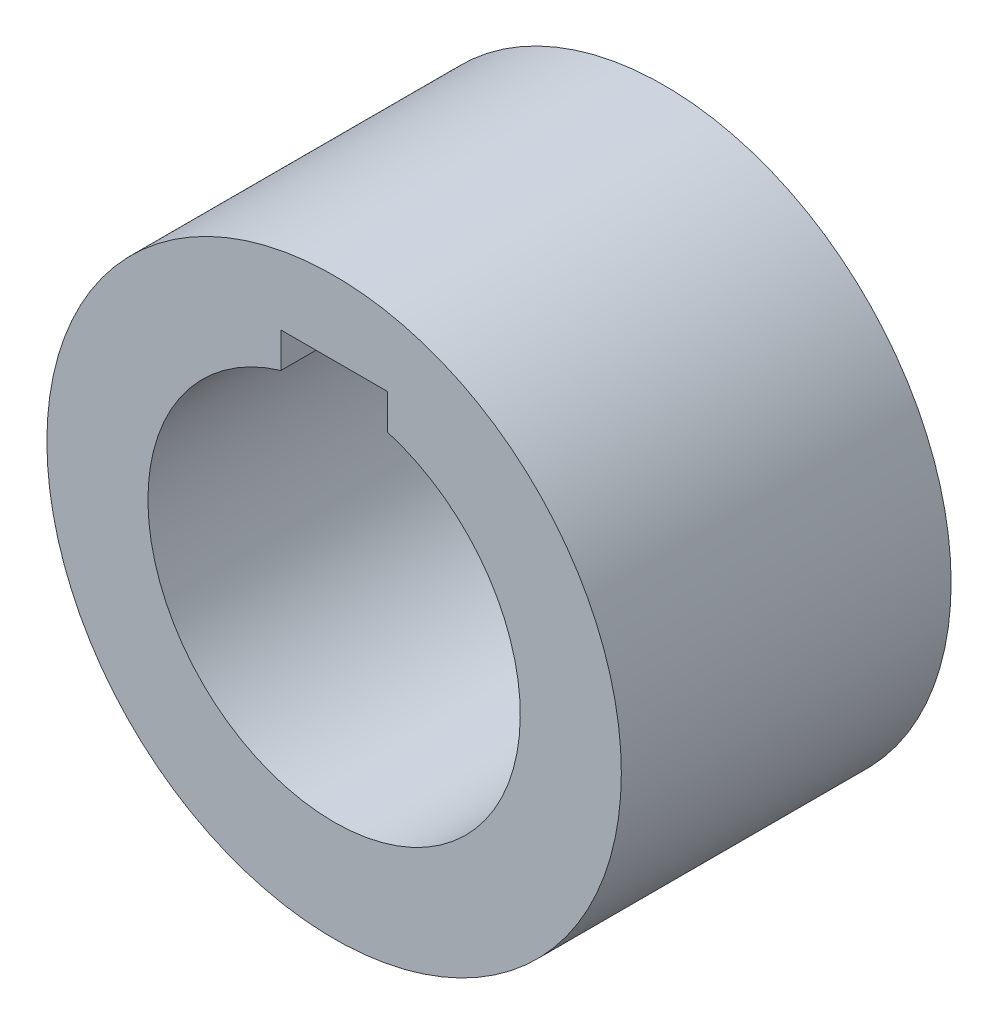
from build123d import *

# Parameters (mm, degrees)
SKETCH_1_R               = 32
EXTRUDE_1_DEPTH          = 31
CUT_EXTRUDE_1_DEPTH      = 55.854352608
PATTERN_CIRCULAR_1_COUNT = 30
CUT_EXTRUDE_2_DEPTH      = 55.792153984
SKETCH_5_OUTSIDE_W       = 85.106
SKETCH_5_OUTSIDE_H       = 84.892
SKETCH_5_OUTSIDE_R       = 27
CUT_EXTRUDE_3_DEPTH      = 42


with BuildPart() as part:
    # 草图1 → 凸台-拉伸1 (new body)
    with BuildSketch(Plane.XY):
        Circle(SKETCH_1_R)
    extrude(amount=EXTRUDE_1_DEPTH)

    # 草图2 → 切除-拉伸1 (cut, through all)
    with BuildSketch(Plane.XY):
        with BuildLine():
            ThreePointArc((0.291117258, 27.498459061), (0, 27.5), (-0.291117258, 27.498459061))
            add(Edge.make_bspline(
                [(-0.291117258, 27.498459061), (-1.016461379, 27.62595034), (-1.020609493, 28.094265272), (-1.11796964, 28.57715803), (-1.139901483, 28.676258475), (-1.166494173, 28.785849819), (-1.198135434, 28.905795984), (-1.235261247, 29.035929815), (-1.278286716, 29.176077028), (-1.327627025, 29.326048954), (-1.383690587, 29.485644922), (-1.446880683, 29.65465171), (-1.517594534, 29.8328439), (-1.596223153, 30.019983966), (-1.683150964, 30.215822454), (-1.778755503, 30.42009815), (-1.883407094, 30.632538255), (-1.99746854, 30.852858572), (-2.121294814, 31.0807637), (-2.255232758, 31.315947232), (-2.399620786, 31.558091968), (-2.554788592, 31.806870128), (-2.721056861, 32.061943577), (-2.89873699, 32.322964055), (-3.088130814, 32.589573415), (-3.289530328, 32.861403867), (-3.503217435, 33.138078232), (-3.729463678, 33.419210196), (-3.968529992, 33.70440458), (-4.220666464, 33.993257607), (-4.486112085, 34.285357181), (-4.765094529, 34.580283169), (-5.057829915, 34.877607694), (-5.364522622, 35.176895427), (-5.685364966, 35.47770389), (-6.137847732, 35.885241657), (-6.490689237, 36.184143062), (-6.732623663, 36.381116246)],
                knots=[0, 0, 0, 0, 0.115323882, 0.12341257, 0.132512303, 0.142623081, 0.153744905, 0.165877774, 0.179021689, 0.193176649, 0.208342655, 0.224519706, 0.241707802, 0.259906945, 0.279117132, 0.299338365, 0.320570644, 0.342813968, 0.366068337, 0.390333752, 0.415610213, 0.441897719, 0.46919627, 0.497505867, 0.52682651, 0.557158198, 0.588500931, 0.62085471, 0.654219534, 0.688595404, 0.723982319, 0.76038028, 0.797789286, 0.836209338, 0.875640435, 0.916082578, 1, 1, 1, 1], degree=3))
            ThreePointArc((-6.732623663, 36.381116246), (0, 36.998835667), (6.732623663, 36.381116246))
            add(Edge.make_bspline(
                [(0.291117258, 27.498459061), (1.016461379, 27.62595034), (1.020609493, 28.094265272), (1.11796964, 28.57715803), (1.139901483, 28.676258475), (1.166494173, 28.785849819), (1.198135434, 28.905795984), (1.235261247, 29.035929815), (1.278286716, 29.176077028), (1.327627025, 29.326048954), (1.383690587, 29.485644922), (1.446880683, 29.65465171), (1.517594534, 29.8328439), (1.596223153, 30.019983966), (1.683150964, 30.215822454), (1.778755503, 30.42009815), (1.883407094, 30.632538255), (1.99746854, 30.852858572), (2.121294814, 31.0807637), (2.255232758, 31.315947232), (2.399620786, 31.558091968), (2.554788592, 31.806870128), (2.721056861, 32.061943577), (2.89873699, 32.322964055), (3.088130814, 32.589573415), (3.289530328, 32.861403867), (3.503217435, 33.138078232), (3.729463678, 33.419210196), (3.968529992, 33.70440458), (4.220666464, 33.993257607), (4.486112085, 34.285357181), (4.765094529, 34.580283169), (5.057829915, 34.877607694), (5.364522622, 35.176895427), (5.685364966, 35.47770389), (6.137847732, 35.885241657), (6.490689237, 36.184143062), (6.732623663, 36.381116246)],
                knots=[0, 0, 0, 0, 0.115323882, 0.12341257, 0.132512303, 0.142623081, 0.153744905, 0.165877774, 0.179021689, 0.193176649, 0.208342655, 0.224519706, 0.241707802, 0.259906945, 0.279117132, 0.299338365, 0.320570644, 0.342813968, 0.366068337, 0.390333752, 0.415610213, 0.441897719, 0.46919627, 0.497505867, 0.52682651, 0.557158198, 0.588500931, 0.62085471, 0.654219534, 0.688595404, 0.723982319, 0.76038028, 0.797789286, 0.836209338, 0.875640435, 0.916082578, 1, 1, 1, 1], degree=3))
        make_face()
    cut_extrude_1 = extrude(amount=CUT_EXTRUDE_1_DEPTH, mode=Mode.SUBTRACT)

    # 阵列(圆周)1: 切除-拉伸1 ×30 about axis
    pattern_circular_1_axis = Axis((0, 0, 31), (0, 0, -1))
    for i in range(1, PATTERN_CIRCULAR_1_COUNT):
        add(cut_extrude_1.rotate(pattern_circular_1_axis, i * 360 / PATTERN_CIRCULAR_1_COUNT), mode=Mode.SUBTRACT)

    # 草图4 → 切除-拉伸2 (cut, through all)
    with BuildSketch(Plane.XY.offset(31)):
        with BuildLine():
            Line((5, 16.770509831), (5, 20.070509831))
            Line((5, 20.070509831), (-5, 20.070509831))
            Line((-5, 20.070509831), (-5, 16.770509831))
            ThreePointArc((-5, 16.770509831), (0, -17.5), (5, 16.770509831))
        make_face()
    extrude(amount=-CUT_EXTRUDE_2_DEPTH, mode=Mode.SUBTRACT)

    # 草图5 outside → 切除-拉伸3 (cut)
    with BuildSketch(Plane.XY):
        Rectangle(SKETCH_5_OUTSIDE_W, SKETCH_5_OUTSIDE_H)
        Circle(SKETCH_5_OUTSIDE_R, mode=Mode.SUBTRACT)
    extrude(amount=CUT_EXTRUDE_3_DEPTH, mode=Mode.SUBTRACT)


solid = part.part
